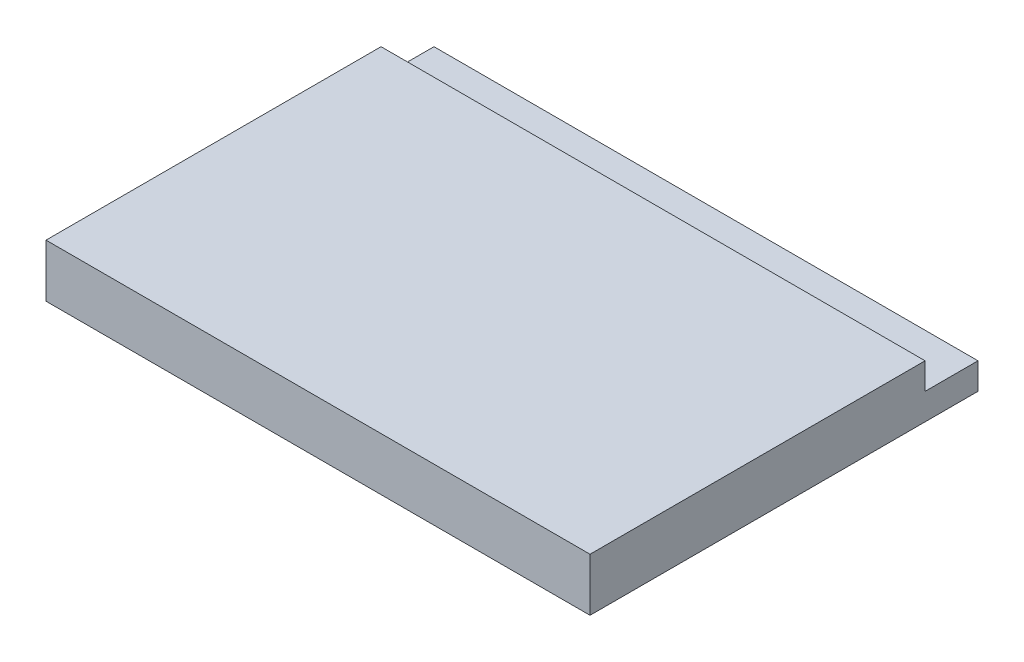
from build123d import *

# Parameters (mm, degrees)
SKETCH_1_W          = 308.5
SKETCH_1_H          = 220
EXTRUDE_1_DEPTH     = 30
SKETCH_2_W          = 366.462982974
SKETCH_2_H          = 68.169207718
CUT_EXTRUDE_1_DEPTH = 15


with BuildPart() as part:
    # 草图1 → 凸台-拉伸1 (new body)
    with BuildSketch(Plane(origin=(0, 0, 0), x_dir=(1, 0, 0), z_dir=(0, 1, 0))):
        Rectangle(SKETCH_1_W, SKETCH_1_H)
    extrude(amount=EXTRUDE_1_DEPTH)

    # 草图2 → 切除-拉伸1 (cut)
    with BuildSketch(Plane(origin=(0, 30, 0), x_dir=(1, 0, 0), z_dir=(0, 1, 0))):
        with Locations((15.777271283, 114.084603859)):
            Rectangle(SKETCH_2_W, SKETCH_2_H)
    extrude(amount=-CUT_EXTRUDE_1_DEPTH, mode=Mode.SUBTRACT)


solid = part.part
